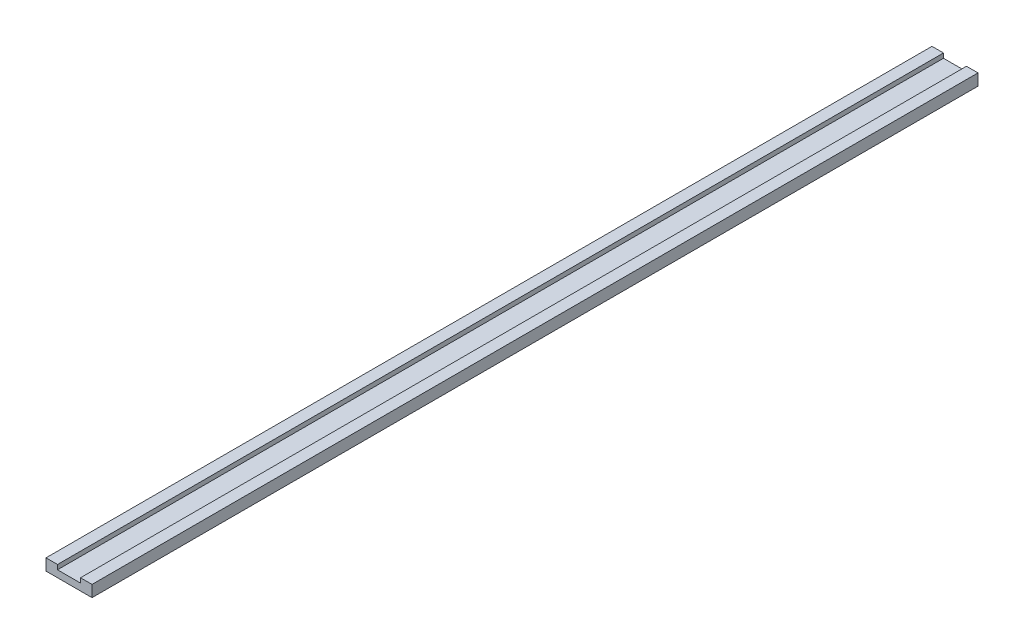
from build123d import *

# Parameters (mm, degrees)
BOSS_EXTRUDE1_DEPTH = 385


with BuildPart() as part:
    # Sketch1 → Boss-Extrude1 (new body)
    with BuildSketch(Plane.XY):
        Polygon((5, 5), (5, 3), (15, 3), (15, 5), (20, 5), (20, 0), (0, 0), (0, 5), align=None)
    extrude(amount=BOSS_EXTRUDE1_DEPTH)


solid = part.part
